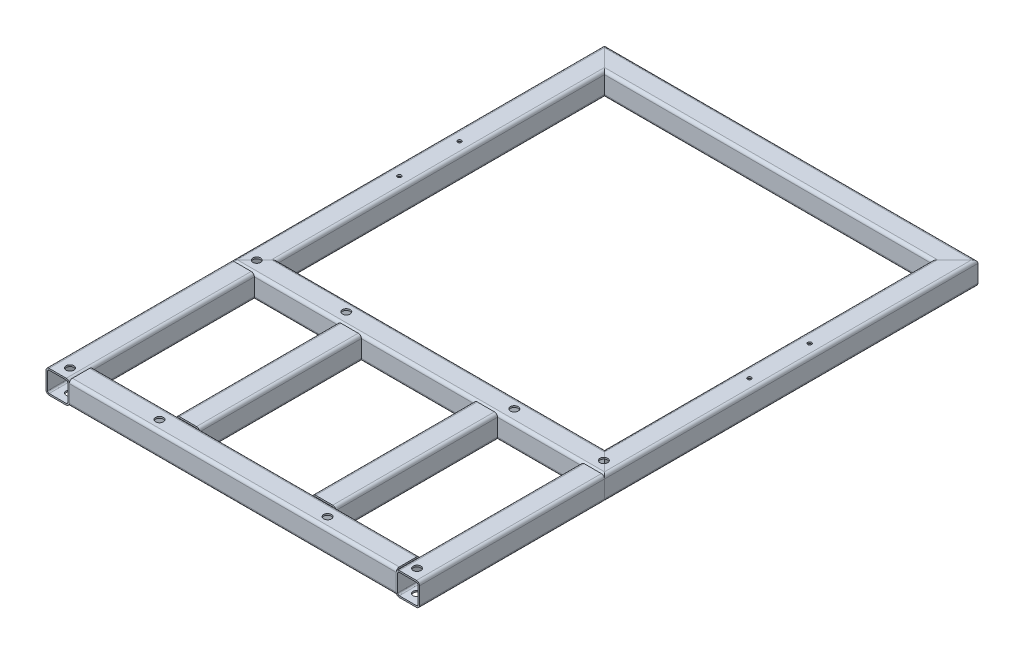
from build123d import *

# Parameters (mm, degrees)
GB_6728_1986_060_X_60_X_4_1_DEPTH      = 943.426406871
GB_6728_1986_060_X_60_X_4_1_DEPTH_BACK = 43.426406871
GB_6728_1986_060_X_60_X_4_1_2_DEPTH    = 986.852813742
GB_6728_1986_060_X_60_X_4_1_3_DEPTH    = 986.852813742
GB_6728_1986_060_X_60_X_4_1_4_DEPTH    = 986.852813742
GB_6728_1986_060_X_60_X_4_1_5_DEPTH    = 477.5
GB_6728_1986_060_X_60_X_4_1_6_DEPTH    = 477.5
GB_6728_1986_060_X_60_X_4_1_7_DEPTH    = 506.5
GB_6728_1986_060_X_60_X_4_1_8_DEPTH    = 506.5
GB_6728_1986_060_X_60_X_4_1_9_DEPTH    = 902
SKETCH_2_R                             = 5
CUT_EXTRUDE_1_DEPTH                    = 90
SKETCH_7_R                             = 10
CUT_EXTRUDE_2_DEPTH                    = 400
PATTERN_LINEAR_1_COUNT                 = 2
PATTERN_LINEAR_1_PITCH                 = 230
MIRROR_3_COPY_1_SKETCH_R               = 10
MIRROR_3_COPY_1_DEPTH                  = 400
MIRROR_4_COPY_1_SKETCH_R               = 10
MIRROR_4_COPY_1_DEPTH                  = 400
MIRROR_4_COPY_2_SKETCH_R               = 10
MIRROR_4_COPY_2_DEPTH                  = 400
MIRROR_4_COPY_3_SKETCH_R               = 10
MIRROR_4_COPY_3_DEPTH                  = 400


with BuildPart() as part:
    # Sketch127 → Gb／6728-1986方形空心型钢 060 X 60 X 4(1) (new, two sides: drawn at the far end of the back side and taken through both)
    with BuildSketch(Plane(origin=(-450, 0, 450), x_dir=(-1, 0, 0), z_dir=(0, 0, -1)).offset(-GB_6728_1986_060_X_60_X_4_1_DEPTH_BACK)):
        with BuildLine():
            Line((-22, -30), (22, -30))
            ThreePointArc((22, -30), (27.656854249, -27.656854249), (30, -22))
            Line((30, -22), (30, 22))
            ThreePointArc((30, 22), (27.656854249, 27.656854249), (22, 30))
            Line((22, 30), (-22, 30))
            ThreePointArc((-22, 30), (-27.656854249, 27.656854249), (-30, 22))
            Line((-30, 22), (-30, -22))
            ThreePointArc((-30, -22), (-27.656854249, -27.656854249), (-22, -30))
        make_face()
        with BuildLine():
            Line((-22, -26), (22, -26))
            ThreePointArc((22, -26), (24.828427125, -24.828427125), (26, -22))
            Line((26, -22), (26, 22))
            ThreePointArc((26, 22), (24.828427125, 24.828427125), (22, 26))
            Line((22, 26), (-22, 26))
            ThreePointArc((-22, 26), (-24.828427125, 24.828427125), (-26, 22))
            Line((-26, 22), (-26, -22))
            ThreePointArc((-26, -22), (-24.828427125, -24.828427125), (-22, -26))
        make_face(mode=Mode.SUBTRACT)
    extrude(amount=GB_6728_1986_060_X_60_X_4_1_DEPTH + GB_6728_1986_060_X_60_X_4_1_DEPTH_BACK)

    # Gb／6728-1986方形空心型钢 060 X 60 X 4(1) mitre 1
    split(bisect_by=Plane(origin=(-450, 0, 450), x_dir=(0, -1, 0), z_dir=(-0.707106781, 0, -0.707106781)), keep=Keep.TOP)

    # Gb／6728-1986方形空心型钢 060 X 60 X 4(1) mitre 2
    split(bisect_by=Plane(origin=(-450, 0, -450), x_dir=(0, -1, 0), z_dir=(-0.707106781, 0, 0.707106781)), keep=Keep.TOP)


with BuildPart() as body_2:
    # Sketch127 on segment 2 (carried to segment 2) → Gb_6728-1986_ 060 X 60 X 4_1 2 (new body)
    with BuildSketch(Plane(origin=(-493.426406871, 0, -450), x_dir=(0, 0, -1), z_dir=(1, 0, 0))):
        with BuildLine():
            Line((-22, -30), (22, -30))
            ThreePointArc((22, -30), (27.656854249, -27.656854249), (30, -22))
            Line((30, -22), (30, 22))
            ThreePointArc((30, 22), (27.656854249, 27.656854249), (22, 30))
            Line((22, 30), (-22, 30))
            ThreePointArc((-22, 30), (-27.656854249, 27.656854249), (-30, 22))
            Line((-30, 22), (-30, -22))
            ThreePointArc((-30, -22), (-27.656854249, -27.656854249), (-22, -30))
        make_face()
        with BuildLine():
            Line((-22, -26), (22, -26))
            ThreePointArc((22, -26), (24.828427125, -24.828427125), (26, -22))
            Line((26, -22), (26, 22))
            ThreePointArc((26, 22), (24.828427125, 24.828427125), (22, 26))
            Line((22, 26), (-22, 26))
            ThreePointArc((-22, 26), (-24.828427125, 24.828427125), (-26, 22))
            Line((-26, 22), (-26, -22))
            ThreePointArc((-26, -22), (-24.828427125, -24.828427125), (-22, -26))
        make_face(mode=Mode.SUBTRACT)
    extrude(amount=GB_6728_1986_060_X_60_X_4_1_2_DEPTH)

    # Gb_6728-1986_ 060 X 60 X 4_1 2 mitre 1
    split(bisect_by=Plane(origin=(-450, 0, -450), x_dir=(0, 1, 0), z_dir=(0.707106781, 0, -0.707106781)), keep=Keep.TOP)

    # Gb_6728-1986_ 060 X 60 X 4_1 2 mitre 2
    split(bisect_by=Plane(origin=(450, 0, -450), x_dir=(0, -1, 0), z_dir=(-0.707106781, 0, -0.707106781)), keep=Keep.TOP)


with BuildPart() as body_3:
    # Sketch127 on segment 3 (carried to segment 3) → Gb_6728-1986_ 060 X 60 X 4_1 3 (new body)
    with BuildSketch(Plane(origin=(450, 0, -493.426406871), x_dir=(1, 0, 0), z_dir=(0, 0, 1))):
        with BuildLine():
            Line((-22, -30), (22, -30))
            ThreePointArc((22, -30), (27.656854249, -27.656854249), (30, -22))
            Line((30, -22), (30, 22))
            ThreePointArc((30, 22), (27.656854249, 27.656854249), (22, 30))
            Line((22, 30), (-22, 30))
            ThreePointArc((-22, 30), (-27.656854249, 27.656854249), (-30, 22))
            Line((-30, 22), (-30, -22))
            ThreePointArc((-30, -22), (-27.656854249, -27.656854249), (-22, -30))
        make_face()
        with BuildLine():
            Line((-22, -26), (22, -26))
            ThreePointArc((22, -26), (24.828427125, -24.828427125), (26, -22))
            Line((26, -22), (26, 22))
            ThreePointArc((26, 22), (24.828427125, 24.828427125), (22, 26))
            Line((22, 26), (-22, 26))
            ThreePointArc((-22, 26), (-24.828427125, 24.828427125), (-26, 22))
            Line((-26, 22), (-26, -22))
            ThreePointArc((-26, -22), (-24.828427125, -24.828427125), (-22, -26))
        make_face(mode=Mode.SUBTRACT)
    extrude(amount=GB_6728_1986_060_X_60_X_4_1_3_DEPTH)

    # Gb_6728-1986_ 060 X 60 X 4_1 3 mitre 1
    split(bisect_by=Plane(origin=(450, 0, 450), x_dir=(0, 1, 0), z_dir=(0.707106781, 0, -0.707106781)), keep=Keep.TOP)

    # Gb_6728-1986_ 060 X 60 X 4_1 3 mitre 2
    split(bisect_by=Plane(origin=(450, 0, -450), x_dir=(0, 1, 0), z_dir=(0.707106781, 0, 0.707106781)), keep=Keep.TOP)


with BuildPart() as body_4:
    # Sketch127 on segment 4 (carried to segment 4) → Gb_6728-1986_ 060 X 60 X 4_1 4 (new body)
    with BuildSketch(Plane(origin=(493.426406871, 0, 450), x_dir=(0, 0, 1), z_dir=(-1, 0, 0))):
        with BuildLine():
            Line((-22, -30), (22, -30))
            ThreePointArc((22, -30), (27.656854249, -27.656854249), (30, -22))
            Line((30, -22), (30, 22))
            ThreePointArc((30, 22), (27.656854249, 27.656854249), (22, 30))
            Line((22, 30), (-22, 30))
            ThreePointArc((-22, 30), (-27.656854249, 27.656854249), (-30, 22))
            Line((-30, 22), (-30, -22))
            ThreePointArc((-30, -22), (-27.656854249, -27.656854249), (-22, -30))
        make_face()
        with BuildLine():
            Line((-22, -26), (22, -26))
            ThreePointArc((22, -26), (24.828427125, -24.828427125), (26, -22))
            Line((26, -22), (26, 22))
            ThreePointArc((26, 22), (24.828427125, 24.828427125), (22, 26))
            Line((22, 26), (-22, 26))
            ThreePointArc((-22, 26), (-24.828427125, 24.828427125), (-26, 22))
            Line((-26, 22), (-26, -22))
            ThreePointArc((-26, -22), (-24.828427125, -24.828427125), (-22, -26))
        make_face(mode=Mode.SUBTRACT)
    extrude(amount=GB_6728_1986_060_X_60_X_4_1_4_DEPTH)

    # Gb_6728-1986_ 060 X 60 X 4_1 4 mitre 1
    split(bisect_by=Plane(origin=(-450, 0, 450), x_dir=(0, 1, 0), z_dir=(0.707106781, 0, 0.707106781)), keep=Keep.TOP)

    # Gb_6728-1986_ 060 X 60 X 4_1 4 mitre 2
    split(bisect_by=Plane(origin=(450, 0, 450), x_dir=(0, -1, 0), z_dir=(-0.707106781, 0, 0.707106781)), keep=Keep.TOP)


with BuildPart() as body_5:
    # Sketch127 on segment 5 (carried to segment 5) → Gb_6728-1986_ 060 X 60 X 4_1 5 (new body)
    with BuildSketch(Plane(origin=(-175, 0, 449), x_dir=(1, 0, 0), z_dir=(0, 0, 1))):
        with BuildLine():
            Line((-22, -30), (22, -30))
            ThreePointArc((22, -30), (27.656854249, -27.656854249), (30, -22))
            Line((30, -22), (30, 22))
            ThreePointArc((30, 22), (27.656854249, 27.656854249), (22, 30))
            Line((22, 30), (-22, 30))
            ThreePointArc((-22, 30), (-27.656854249, 27.656854249), (-30, 22))
            Line((-30, 22), (-30, -22))
            ThreePointArc((-30, -22), (-27.656854249, -27.656854249), (-22, -30))
        make_face()
        with BuildLine():
            Line((-22, -26), (22, -26))
            ThreePointArc((22, -26), (24.828427125, -24.828427125), (26, -22))
            Line((26, -22), (26, 22))
            ThreePointArc((26, 22), (24.828427125, 24.828427125), (22, 26))
            Line((22, 26), (-22, 26))
            ThreePointArc((-22, 26), (-24.828427125, 24.828427125), (-26, 22))
            Line((-26, 22), (-26, -22))
            ThreePointArc((-26, -22), (-24.828427125, -24.828427125), (-22, -26))
        make_face(mode=Mode.SUBTRACT)
    extrude(amount=GB_6728_1986_060_X_60_X_4_1_5_DEPTH)

    # Gb_6728-1986_ 060 X 60 X 4_1 5 mitre 1
    split(bisect_by=Plane(origin=(-175, 0, 480), x_dir=(0, -1, 0), z_dir=(0, 0, 1)), keep=Keep.TOP)

    # Gb_6728-1986_ 060 X 60 X 4_1 5 mitre 2
    split(bisect_by=Plane(origin=(-175, 0, 895.5), x_dir=(0, 1, 0), z_dir=(0, 0, -1)), keep=Keep.TOP)


with BuildPart() as body_6:
    # Sketch127 on segment 6 (carried to segment 6) → Gb_6728-1986_ 060 X 60 X 4_1 6 (new body)
    with BuildSketch(Plane(origin=(175, 0, 449), x_dir=(1, 0, 0), z_dir=(0, 0, 1))):
        with BuildLine():
            Line((-22, -30), (22, -30))
            ThreePointArc((22, -30), (27.656854249, -27.656854249), (30, -22))
            Line((30, -22), (30, 22))
            ThreePointArc((30, 22), (27.656854249, 27.656854249), (22, 30))
            Line((22, 30), (-22, 30))
            ThreePointArc((-22, 30), (-27.656854249, 27.656854249), (-30, 22))
            Line((-30, 22), (-30, -22))
            ThreePointArc((-30, -22), (-27.656854249, -27.656854249), (-22, -30))
        make_face()
        with BuildLine():
            Line((-22, -26), (22, -26))
            ThreePointArc((22, -26), (24.828427125, -24.828427125), (26, -22))
            Line((26, -22), (26, 22))
            ThreePointArc((26, 22), (24.828427125, 24.828427125), (22, 26))
            Line((22, 26), (-22, 26))
            ThreePointArc((-22, 26), (-24.828427125, 24.828427125), (-26, 22))
            Line((-26, 22), (-26, -22))
            ThreePointArc((-26, -22), (-24.828427125, -24.828427125), (-22, -26))
        make_face(mode=Mode.SUBTRACT)
    extrude(amount=GB_6728_1986_060_X_60_X_4_1_6_DEPTH)

    # Gb_6728-1986_ 060 X 60 X 4_1 6 mitre 1
    split(bisect_by=Plane(origin=(175, 0, 480), x_dir=(0, -1, 0), z_dir=(0, 0, 1)), keep=Keep.TOP)

    # Gb_6728-1986_ 060 X 60 X 4_1 6 mitre 2
    split(bisect_by=Plane(origin=(175, 0, 895.5), x_dir=(0, 1, 0), z_dir=(0, 0, -1)), keep=Keep.TOP)


with BuildPart() as body_7:
    # Sketch127 on segment 7 (carried to segment 7) → Gb_6728-1986_ 060 X 60 X 4_1 7 (new body)
    with BuildSketch(Plane(origin=(-450, 0, 449), x_dir=(1, 0, 0), z_dir=(0, 0, 1))):
        with BuildLine():
            Line((-22, -30), (22, -30))
            ThreePointArc((22, -30), (27.656854249, -27.656854249), (30, -22))
            Line((30, -22), (30, 22))
            ThreePointArc((30, 22), (27.656854249, 27.656854249), (22, 30))
            Line((22, 30), (-22, 30))
            ThreePointArc((-22, 30), (-27.656854249, 27.656854249), (-30, 22))
            Line((-30, 22), (-30, -22))
            ThreePointArc((-30, -22), (-27.656854249, -27.656854249), (-22, -30))
        make_face()
        with BuildLine():
            Line((-22, -26), (22, -26))
            ThreePointArc((22, -26), (24.828427125, -24.828427125), (26, -22))
            Line((26, -22), (26, 22))
            ThreePointArc((26, 22), (24.828427125, 24.828427125), (22, 26))
            Line((22, 26), (-22, 26))
            ThreePointArc((-22, 26), (-24.828427125, 24.828427125), (-26, 22))
            Line((-26, 22), (-26, -22))
            ThreePointArc((-26, -22), (-24.828427125, -24.828427125), (-22, -26))
        make_face(mode=Mode.SUBTRACT)
    extrude(amount=GB_6728_1986_060_X_60_X_4_1_7_DEPTH)

    # Gb_6728-1986_ 060 X 60 X 4_1 7 mitre 1
    split(bisect_by=Plane(origin=(-450, 0, 480), x_dir=(0, -1, 0), z_dir=(0, 0, 1)), keep=Keep.TOP)


with BuildPart() as body_8:
    # Sketch127 on segment 8 (carried to segment 8) → Gb_6728-1986_ 060 X 60 X 4_1 8 (new body)
    with BuildSketch(Plane(origin=(450, 0, 955.5), x_dir=(-1, 0, 0), z_dir=(0, 0, -1))):
        with BuildLine():
            Line((-22, -30), (22, -30))
            ThreePointArc((22, -30), (27.656854249, -27.656854249), (30, -22))
            Line((30, -22), (30, 22))
            ThreePointArc((30, 22), (27.656854249, 27.656854249), (22, 30))
            Line((22, 30), (-22, 30))
            ThreePointArc((-22, 30), (-27.656854249, 27.656854249), (-30, 22))
            Line((-30, 22), (-30, -22))
            ThreePointArc((-30, -22), (-27.656854249, -27.656854249), (-22, -30))
        make_face()
        with BuildLine():
            Line((-22, -26), (22, -26))
            ThreePointArc((22, -26), (24.828427125, -24.828427125), (26, -22))
            Line((26, -22), (26, 22))
            ThreePointArc((26, 22), (24.828427125, 24.828427125), (22, 26))
            Line((22, 26), (-22, 26))
            ThreePointArc((-22, 26), (-24.828427125, 24.828427125), (-26, 22))
            Line((-26, 22), (-26, -22))
            ThreePointArc((-26, -22), (-24.828427125, -24.828427125), (-22, -26))
        make_face(mode=Mode.SUBTRACT)
    extrude(amount=GB_6728_1986_060_X_60_X_4_1_8_DEPTH)

    # Gb_6728-1986_ 060 X 60 X 4_1 8 mitre 1
    split(bisect_by=Plane(origin=(450, 0, 480), x_dir=(0, -1, 0), z_dir=(0, 0, 1)), keep=Keep.TOP)

    # 草图7 → 切除-拉伸2 (cut)
    with BuildSketch(Plane(origin=(0, 30, 0), x_dir=(1, 0, 0), z_dir=(0, 1, 0))):
        with Locations(Location((446, -927.75, 0), (0, 0, 270))):
            Circle(SKETCH_7_R)
    cut_extrude_2 = extrude(amount=-CUT_EXTRUDE_2_DEPTH, mode=Mode.SUBTRACT)


with BuildPart() as body_9:
    # Sketch127 on segment 9 (carried to segment 9) → Gb_6728-1986_ 060 X 60 X 4_1 9 (new body)
    with BuildSketch(Plane(origin=(-451, 0, 925.5), x_dir=(0, 0, -1), z_dir=(1, 0, 0))):
        with BuildLine():
            Line((-22, -30), (22, -30))
            ThreePointArc((22, -30), (27.656854249, -27.656854249), (30, -22))
            Line((30, -22), (30, 22))
            ThreePointArc((30, 22), (27.656854249, 27.656854249), (22, 30))
            Line((22, 30), (-22, 30))
            ThreePointArc((-22, 30), (-27.656854249, 27.656854249), (-30, 22))
            Line((-30, 22), (-30, -22))
            ThreePointArc((-30, -22), (-27.656854249, -27.656854249), (-22, -30))
        make_face()
        with BuildLine():
            Line((-22, -26), (22, -26))
            ThreePointArc((22, -26), (24.828427125, -24.828427125), (26, -22))
            Line((26, -22), (26, 22))
            ThreePointArc((26, 22), (24.828427125, 24.828427125), (22, 26))
            Line((22, 26), (-22, 26))
            ThreePointArc((-22, 26), (-24.828427125, 24.828427125), (-26, 22))
            Line((-26, 22), (-26, -22))
            ThreePointArc((-26, -22), (-24.828427125, -24.828427125), (-22, -26))
        make_face(mode=Mode.SUBTRACT)
    extrude(amount=GB_6728_1986_060_X_60_X_4_1_9_DEPTH)

    # Gb_6728-1986_ 060 X 60 X 4_1 9 mitre 1
    split(bisect_by=Plane(origin=(-420, 0, 925.5), x_dir=(0, 1, 0), z_dir=(1, 0, 0)), keep=Keep.TOP)

    # Gb_6728-1986_ 060 X 60 X 4_1 9 mitre 2
    split(bisect_by=Plane(origin=(420, 0, 925.5), x_dir=(0, -1, 0), z_dir=(-1, 0, 0)), keep=Keep.TOP)

    # 阵列(线性)1: 切除-拉伸2 ×2
    with Locations(*[(-i * PATTERN_LINEAR_1_PITCH, 0, 0) for i in range(1, PATTERN_LINEAR_1_COUNT)]):
        add(cut_extrude_2, mode=Mode.SUBTRACT)

    # 镜向3 copy 1 sketch → 镜向3 copy 1 (cut)
    with BuildSketch(Plane(origin=(230, 30, 0), x_dir=(-1, 0, 0), z_dir=(0, 1, 0))):
        with Locations((446, 927.75)):
            Circle(MIRROR_3_COPY_1_SKETCH_R)
    extrude(amount=-MIRROR_3_COPY_1_DEPTH, mode=Mode.SUBTRACT)


with BuildPart() as cut_extrude_1_tool:
    # 草图2 → 切除-拉伸1 (new body)
    with BuildSketch(Plane(origin=(0, 30, 0), x_dir=(1, 0, 0), z_dir=(0, 1, 0))):
        with Locations(Location((450, 77.5, 0), (0, 0, 270))):
            Circle(SKETCH_2_R)
        with Locations(Location((450, -77.5, 0), (0, 0, 270))):
            Circle(SKETCH_2_R)
        with Locations(Location((-450, -77.5, 0), (0, 0, 270))):
            Circle(SKETCH_2_R)
        with Locations(Location((-450, 77.5, 0), (0, 0, 270))):
            Circle(SKETCH_2_R)
    extrude(amount=-CUT_EXTRUDE_1_DEPTH)


with BuildPart() as part_1:
    add(part.part)

    # 切除-拉伸1: cut by cut_extrude_1_tool
    add(cut_extrude_1_tool.part, mode=Mode.SUBTRACT)


with BuildPart() as body_3_1:
    add(body_3.part)

    # 切除-拉伸1: cut by cut_extrude_1_tool
    add(cut_extrude_1_tool.part, mode=Mode.SUBTRACT)


with BuildPart() as body_7_1:
    add(body_7.part)

    # 镜向3: 切除-拉伸2 across plane
    add(cut_extrude_2.mirror(Plane(origin=(0, 0, 0), x_dir=(0, 0, 1), z_dir=(1, 0, 0))), mode=Mode.SUBTRACT)


with BuildPart() as mirror_4_tool:
    # 镜向4: 切除-拉伸2 across plane
    add(cut_extrude_2.mirror(Plane.XY.offset(687.75)))


with BuildPart() as body_3_2:
    add(body_3_1.part)

    # 镜向4: cut by mirror_4_tool
    add(mirror_4_tool.part, mode=Mode.SUBTRACT)


with BuildPart() as body_4_1:
    add(body_4.part)

    # 镜向4: cut by mirror_4_tool
    add(mirror_4_tool.part, mode=Mode.SUBTRACT)

    # 镜向4 copy 1 sketch → 镜向4 copy 1 (cut)
    with BuildSketch(Plane(origin=(-230, 30, 1375.5), x_dir=(1, 0, 0), z_dir=(0, 1, 0))):
        with Locations((446, 927.75)):
            Circle(MIRROR_4_COPY_1_SKETCH_R)
    extrude(amount=-MIRROR_4_COPY_1_DEPTH, mode=Mode.SUBTRACT)


with BuildPart() as mirror_4_copy_2_tool:
    # 镜向4 copy 2 sketch → 镜向4 copy 2 (new body)
    with BuildSketch(Plane(origin=(0, 30, 1375.5), x_dir=(-1, 0, 0), z_dir=(0, 1, 0))):
        with Locations(Location((446, -927.75, 0), (0, 0, 270))):
            Circle(MIRROR_4_COPY_2_SKETCH_R)
    extrude(amount=-MIRROR_4_COPY_2_DEPTH)


with BuildPart() as part_2:
    add(part_1.part)

    # 镜向4 copy 2: cut by mirror_4_copy_2_tool
    add(mirror_4_copy_2_tool.part, mode=Mode.SUBTRACT)


with BuildPart() as body_4_2:
    add(body_4_1.part)

    # 镜向4 copy 2: cut by mirror_4_copy_2_tool
    add(mirror_4_copy_2_tool.part, mode=Mode.SUBTRACT)

    # 镜向4 copy 3 sketch → 镜向4 copy 3 (cut)
    with BuildSketch(Plane(origin=(230, 30, 1375.5), x_dir=(-1, 0, 0), z_dir=(0, 1, 0))):
        with Locations(Location((446, -927.75, 0), (0, 0, 270))):
            Circle(MIRROR_4_COPY_3_SKETCH_R)
    extrude(amount=-MIRROR_4_COPY_3_DEPTH, mode=Mode.SUBTRACT)


solid = Compound([body_2.part, body_5.part, body_6.part, body_8.part, body_9.part, body_7_1.part, body_3_2.part, part_2.part, body_4_2.part])
